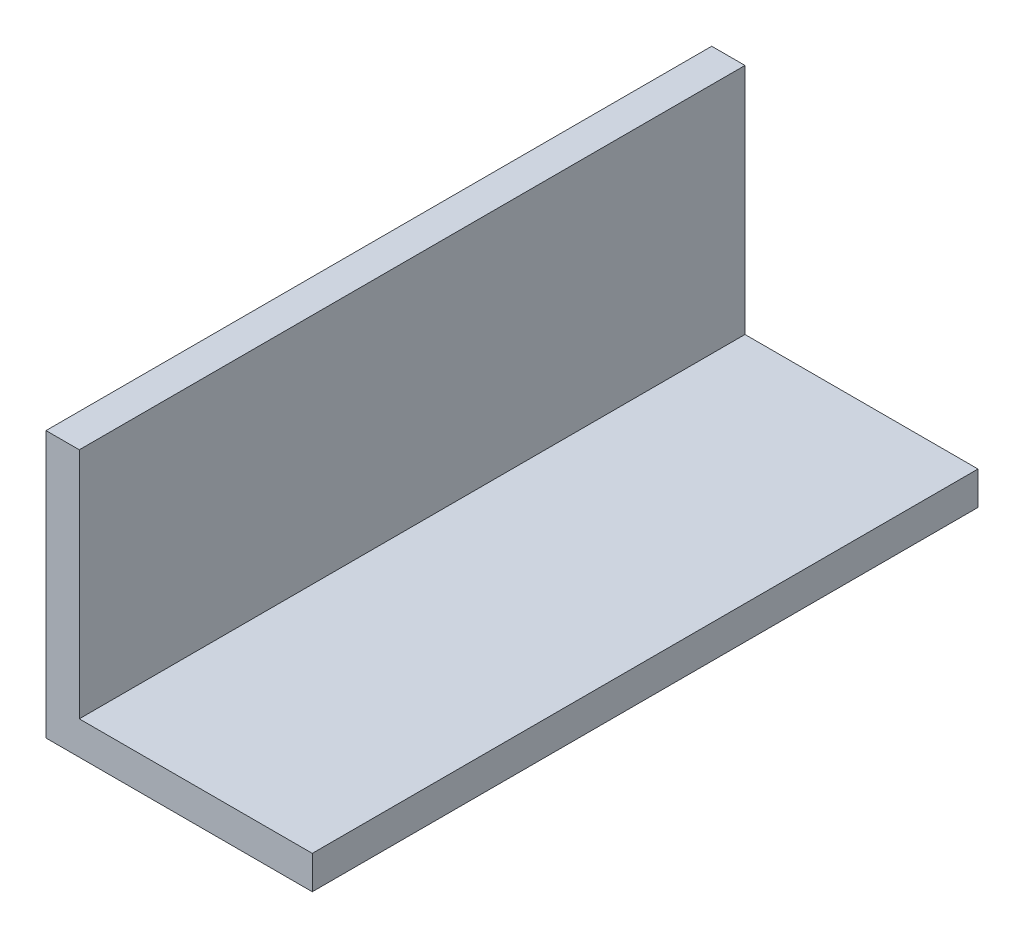
SolidWorks part; units mm, degrees
ref_plane "前视基准面" through (0, 0, 0) normal (0, 0, 1) x (1, 0, 0)
ref_plane "上视基准面" through (0, 0, 0) normal (0, 1, 0) x (1, 0, 0)
ref_plane "右视基准面" through (0, 0, 0) normal (1, 0, 0) x (0, 0, -1)
sketch "草图1" plane through (0, 0, 0) normal (0, 0, 1) x (1, 0, 0)
  line L0 (0, 0) -> (0, -40)
  line L1 (0, -40) -> (40, -40)
  line L2 (5, 0) -> (5, -35)
  line L3 (5, -35) -> (40, -35)
  line L4 (0, 0) -> (5, 0)
  line L5 (40, -40) -> (40, -35)
  dimension "D1" = 5
extrude "凸台-拉伸1" add sketch "草图1" along normal blind 100
